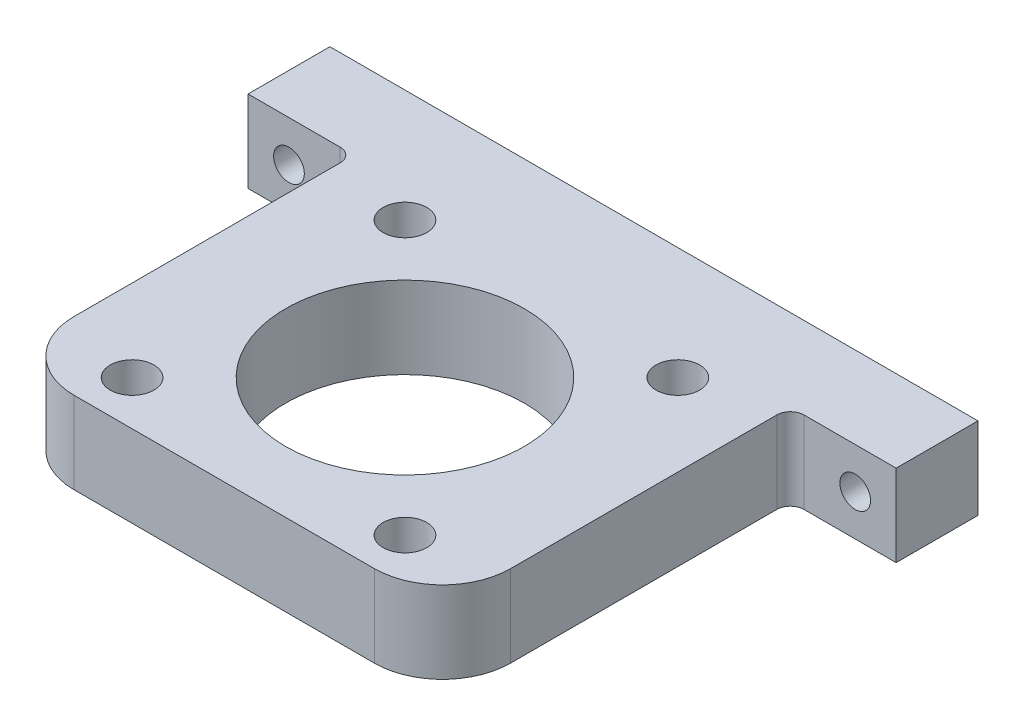
SolidWorks part; units mm, degrees
material "45钢"
ref_plane "前视基准面" through (0, 0, 0) normal (0, 0, 1) x (1, 0, 0)
ref_plane "上视基准面" through (0, 0, 0) normal (0, 1, 0) x (1, 0, 0)
ref_plane "右视基准面" through (0, 0, 0) normal (1, 0, 0) x (0, 0, -1)
sketch "草图1" plane through (0, 0, 0) normal (0, 1, 0) x (1, 0, 0)
  line L0 (0, 0) -> (95, 0)
  line L1 (95, 0) -> (95, -63)
  line L4 (95, -63) -> (0, -63)
  line L5 (0, -63) -> (0, 0)
  dimension "D1" = 95
  dimension "D2" = 63
extrude "凸台-拉伸1" add sketch "草图1" along normal blind 12
hole_wizard "Ø16.0 (16) 直径孔1" positions "草图6" profile "草图5" hole size "Ø16.0" standard "GB"
sketch "草图6" plane through (0, 15, 0) normal (0, 1, 0) x (1, 0, 0)
  line L0 (70, 0) -> (0, 0) construction
  line L2 (35, -31) -> (35, -52) construction
  line L3 (0, -52) -> (70, -52) construction
  point P0 (35, -31)
  dimension "D1" = 31
sketch "草图5" plane through (35, 15, 31) normal (1, 0, 0) x (0, 0, 1)
  line L0 (0, 0) -> (0, 15)
  line L1 (0, 15) -> (8.1, 15)
  line L2 (8.1, 15) -> (8.1, 0)
  line L5 (8.1, 0) -> (0, 0)
  line L11 (0, -6.35) -> (0, 107.95) construction
  dimension "通孔孔直径" = 16.2
  dimension "通孔孔深度" = 15
sketch "草图8" [suppressed] plane through (0, 0, 0) normal (0, -1, 0) x (1, 0, 0)
  line L1 (-59.908, 80.8452) -> (106.3415, 80.8452)
  line L2 (-59.908, 80.8452) -> (-59.908, 14)
  line L3 (-59.908, 14) -> (106.3415, 14)
  line L4 (106.3415, 80.8452) -> (106.3415, 14)
  line L5 (-59.908, 80.8452) -> (106.3415, 14) construction
  line L6 (-59.908, 14) -> (106.3415, 80.8452) construction
  circle A0 centre (35, 31) radius 8.1 construction
  point P0 (23.2167, 47.4226)
  dimension "D1" = 17
extrude "切除-拉伸3" [suppressed] cut sketch "草图8" against normal offset from surface (6 mm away) 9
ref_plane "基准面1" through (47.5, 0, 0) normal (-1, 0, 0) x (0, 0, 1)
sketch "草图9" plane through (0, 12, 0) normal (0, 1, 0) x (1, 0, 0)
  line L0 (95, 0) -> (0, 0) construction
  line L1 (0, -63) -> (15.5, -63)
  line L2 (0, -63) -> (0, -12)
  line L3 (0, -12) -> (15.5, -12)
  line L4 (15.5, -63) -> (15.5, -12)
  line L5 (95, -63) -> (79.5, -63)
  line L6 (95, -63) -> (95, -12)
  line L7 (95, -12) -> (79.5, -12)
  line L8 (79.5, -63) -> (79.5, -12)
  dimension "D1" = 64
  dimension "D2" = 12
extrude "切除-拉伸4" cut sketch "草图9" against normal through all
hole_wizard "Ø6.5 (6.5) 直径孔1" positions "草图10" profile "草图11" hole size "Ø6.5" standard "GB" end condition through all
sketch "草图10" plane through (0, 0, 12) normal (0, 0, 1) x (1, 0, 0)
  line L0 (0, 6) -> (6, 6) construction
  line L1 (0, 0) -> (0, 12) construction
  line L2 (6, 6) -> (89, 6) construction
  line L3 (89, 6) -> (95, 6) construction
  line L4 (95, 0) -> (95, 12) construction
  point P0 (6, 6)
  point P2 (89, 6)
  dimension "D1" = 6
sketch "草图11" plane through (6, 6, 12) normal (1, 0, 0) x (0, -1, 0)
  line L0 (0, 0) -> (0, 12)
  line L1 (0, 12) -> (2.25, 12)
  line L2 (2.25, 12) -> (2.25, 0)
  line L5 (2.25, 0) -> (0, 0)
  line L11 (0, -6.35) -> (0, 107.95) construction
  dimension "通孔孔直径" = 4.5
  dimension "通孔孔深度" = 12
sketch "草图12" plane through (0, 12, 0) normal (0, 1, 0) x (1, 0, 0)
  line L0 (47.5, 0) -> (47.5, -36.5) construction
  line L1 (95, 0) -> (0, 0) construction
  line L2 (15.5, -63) -> (79.5, -63) construction
  circle A0 centre (47.5, -36.5) radius 17.5
  dimension "D2" = 35
  dimension "D1" = 26.5
extrude "切除-拉伸5" cut sketch "草图12" against normal through all
fillet "圆角1" radius 10 2 edges at (15.5, 6, 63) (79.5, 6, 63)
hole_wizard "Ø5.0 (5) 直径孔1" positions "草图13" profile "草图14" hole size "Ø5.0" standard "GB"
sketch "草图13" plane through (0, 0, 0) normal (0, 0, -1) x (-1, 0, 0)
  line L0 (-47.5, 12) -> (-47.5, -2.6375) construction
  line L1 (-95, 12) -> (0, 12) construction
  line L4 (-67.5, 6) -> (-27.5, 6) construction
  line L5 (-27.5, 6) -> (0, 6) construction
  line L6 (0, 12) -> (0, 0) construction
  point P0 (-67.5, 6)
  point P2 (-27.5, 6)
  dimension "D1" = 40
sketch "草图14" plane through (67.5, 6, 0) normal (1, 0, 0) x (0, 1, 0)
  line L0 (0, 0) -> (0, 11.5022)
  line L1 (0, 11.5022) -> (2.5, 10)
  line L2 (2.5, 10) -> (2.5, 0)
  line L5 (2.5, 0) -> (0, 0)
  line L10 (0, 11.5022) -> (-2.5, 10) construction
  line L11 (0, -6.35) -> (0, 107.95) construction
  dimension "孔直径" = 5
  dimension "孔深度" = 10
  dimension "导头角度" = 118
fillet "圆角2" radius 2 2 edges at (15.5, 6, 12) (79.5, 6, 12)
hole_wizard "大小mm 暗销孔1" positions "草图17" profile "草图19" hole size "Ø5.0" standard "GB"
sketch "草图17" plane through (0, 0, 0) normal (0, -1, 0) x (-1, 0, 0)
  point P0 (-72.5, -43)
  point P3 (-72.5, -93)
  point P6 (-22.5, -93)
  point P9 (-22.5, -43)
sketch "草图19" plane through (72.5, 0, 43) normal (1, 0, 0) x (0, 0, -1)
  line L0 (0, 0) -> (0, 12)
  line L1 (0, 12) -> (4.5, 12)
  line L2 (4.5, 12) -> (4.5, 0)
  line L5 (4.5, 0) -> (0, 0)
  line L11 (0, -6.35) -> (0, 107.95) construction
  dimension "通孔孔直径" = 9
  dimension "通孔孔深度" = 12
hole_wizard "M6 螺纹孔1" positions "草图20" profile "草图21" tap size "M6" standard "GB"
sketch "草图20" plane through (0, 0, 0) normal (0, -1, 0) x (-1, 0, 0)
  line L0 (-47.5, -36.5) -> (-47.5, -27.13) construction
  line L1 (-25.5, -63) -> (-69.5, -63) construction
  point P6 (-47.5, -7.5)
  dimension "D1" = 55.5
sketch "草图21" [suppressed] plane through (47.5, 0, 7.5) normal (1, 0, 0) x (0, 0, -1)
  line L0 (0, 0) -> (0, 12)
  line L1 (0, 12) -> (2.5, 12)
  line L2 (2.5, 12) -> (2.5, 0)
  line L5 (2.5, 0) -> (0, 0)
  line L11 (0, -6.35) -> (0, 107.95) construction
  dimension "通孔螺纹孔钻头直径" = 5
  dimension "通孔螺纹孔钻头深度" = 12
cosmetic thread "孔螺蚊线1" parameters "D2"=6
hole_wizard "M6 螺纹孔2" positions "草图23" profile "草图24" tap size "M6" standard "GB"
sketch "草图23" plane through (0, 0, 0) normal (0, -1, 0) x (-1, 0, 0)
  line L0 (-47.5, -20) -> (-47.5, -17) construction
  point P7 (-47.5, -18.5)
sketch "草图24" plane through (47.5, 0, 18.5) normal (1, 0, 0) x (0, 0, -1)
  line L0 (0, 0) -> (0, 12)
  line L1 (0, 12) -> (2.5, 12)
  line L2 (2.5, 12) -> (2.5, 0)
  line L5 (2.5, 0) -> (0, 0)
  line L11 (0, -6.35) -> (0, 107.95) construction
  dimension "通孔螺纹孔钻头直径" = 5
  dimension "通孔螺纹孔钻头深度" = 12
cosmetic thread "孔螺蚊线2" [suppressed] parameters "D2"=6
hole_wizard "打孔尺寸(%根据)内六角圆柱头螺钉的类型1" positions "草图25" profile "草图27" counterbore size "M6" standard "GB" end condition through all
sketch "草图25" plane through (0, 0, 0) normal (0, -1, 0) x (-1, 0, 0)
  point P0 (-67.5, -56.5)
  point P2 (-27.5, -56.5)
  point P4 (-27.5, -16.5)
  point P6 (-67.5, -16.5)
sketch "草图27" plane through (67.5, 0, 56.5) normal (1, 0, 0) x (0, 0, -1)
  line L0 (0, 0) -> (0, 12)
  line L1 (0, 12) -> (3.2, 12)
  line L3 (3.2, 12) -> (3.2, 7)
  line L4 (3.2, 7) -> (5.5, 7)
  line L5 (5.5, 7) -> (5.5, 0)
  line L7 (5.5, 0) -> (0, 0)
  line L11 (0, -6.35) -> (0, 107.95) construction
  dimension "通孔孔直径" = 6.4
  dimension "通孔孔深度" = 12
  dimension "柱形沉头孔直径" = 11
  dimension "柱形沉头孔深度" = 7
